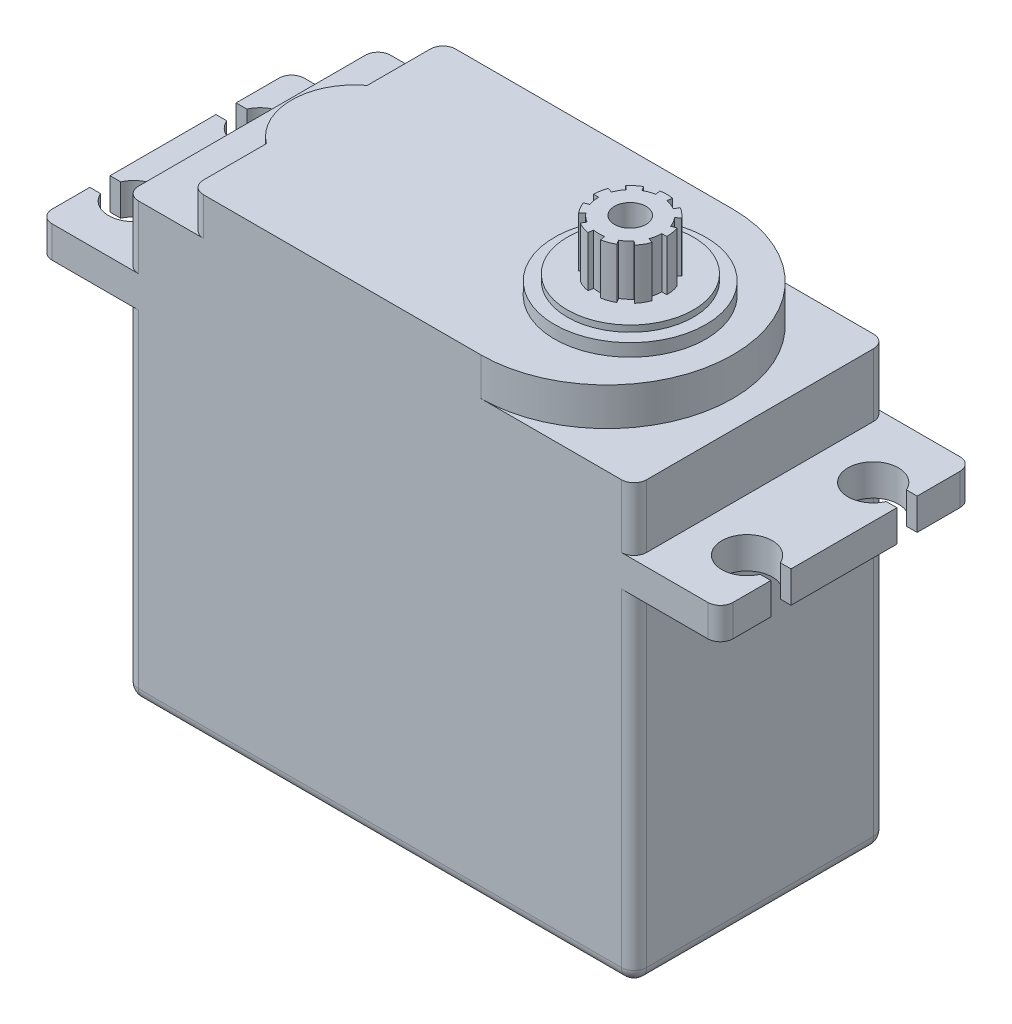
from build123d import *

# Parameters (mm, degrees)
BOSS_EXTRUDE1_DEPTH   = 20
FILLET1_R             = 1
CUT_EXTRUDE1_DEPTH    = 20
SKETCH3_W             = 51.867663345
SKETCH3_H             = 35.261757523
CUT_EXTRUDE2_DEPTH    = 3
SKETCH4_R             = 6
BOSS_EXTRUDE2_DEPTH   = 1
SKETCH5_R             = 5
BOSS_EXTRUDE3_DEPTH   = 0.5
SKETCH6_R             = 1
BOSS_EXTRUDE4_DEPTH   = 4
M3_TAPPED_HOLE1_D     = 2.5
M3_TAPPED_HOLE1_DEPTH = 7.5
M3_TAPPED_HOLE1_TIP   = 0.751075774


with BuildPart() as part:
    # Sketch1 → Boss-Extrude1 (new body)
    with BuildSketch(Plane.XY):
        Polygon((20.15, 8), (27, 8), (27, 10.5), (20.15, 10.5), (20.15, 18.5), (-20.15, 18.5), (-20.15, 10.5), (-27, 10.5), (-27, 8), (-20.15, 8), (-20.15, -19), (20.15, -19), align=None)
    extrude(amount=BOSS_EXTRUDE1_DEPTH)

    # Fillet1
    fillet1_edges = [part.edges().sort_by_distance(p)[0] for p in [
        (-27, 9.25, 20),
        (20.15, 14.5, 0),
        (27, 9.25, 0),
        (20.15, -5.5, 0),
        (0, -19, 0),
        (-20.15, -5.5, 0),
        (-27, 9.25, 0),
        (-20.15, 14.5, 0),
        (-20.15, -5.5, 20),
        (0, -19, 20),
        (-20.15, 18.5, 10),
        (20.15, 18.5, 10),
        (20.15, -19, 10),
        (-20.15, -19, 10),
        (20.15, -5.5, 20),
        (27, 9.25, 20),
        (20.15, 14.5, 20),
        (-20.15, 14.5, 20),
    ]]
    fillet(fillet1_edges, radius=FILLET1_R)

    # Sketch2 → Cut-Extrude1 (cut)
    with BuildSketch(Plane(origin=(0, 10.5, 0), x_dir=(1, 0, 0), z_dir=(0, 1, 0))):
        with BuildLine():
            Line((-26.148030278, -4.4), (-29.222738853, -4.4))
            Line((-29.222738853, -4.4), (-29.222738853, -6))
            Line((-29.222738853, -6), (-26.148030278, -6))
            ThreePointArc((-26.148030278, -6), (-22.315, -5.2), (-26.148030278, -4.4))
        make_face()
        with BuildLine():
            Line((-26.148030278, -14.4), (-29.222738853, -14.4))
            Line((-29.222738853, -14.4), (-29.222738853, -16))
            Line((-29.222738853, -16), (-26.148030278, -16))
            ThreePointArc((-26.148030278, -16), (-22.315, -15.2), (-26.148030278, -14.4))
        make_face()
        with BuildLine():
            Line((26.148030278, -16), (29.222738853, -16))
            Line((29.222738853, -16), (29.222738853, -14.4))
            Line((29.222738853, -14.4), (26.148030278, -14.4))
            ThreePointArc((26.148030278, -14.4), (22.315, -15.2), (26.148030278, -16))
        make_face()
        with BuildLine():
            Line((29.222738853, -4.4), (29.222738853, -6))
            Line((29.222738853, -6), (26.148030278, -6))
            ThreePointArc((26.148030278, -6), (22.315, -5.2), (26.148030278, -4.4))
            Line((26.148030278, -4.4), (29.222738853, -4.4))
        make_face()
    extrude(amount=-CUT_EXTRUDE1_DEPTH, mode=Mode.SUBTRACT)

    # Sketch3 → Cut-Extrude2 (cut)
    with BuildSketch(Plane(origin=(0, 18.5, 0), x_dir=(1, 0, 0), z_dir=(0, 1, 0))):
        with Locations((-0.933831673, -10.85793672)):
            Rectangle(SKETCH3_W, SKETCH3_H)
        with BuildLine():
            Line((-14, 0), (8, 0))
            ThreePointArc((8, 0), (18, -10), (8, -20))
            Line((8, -20), (-14, -20))
            ThreePointArc((-14, -20), (-14.707106781, -19.707106781), (-15, -19))
            Line((-15, -19), (-15, -14))
            ThreePointArc((-15, -14), (-17, -10), (-15, -6))
            Line((-15, -6), (-15, -1))
            ThreePointArc((-15, -1), (-14.707106781, -0.292893219), (-14, 0))
        make_face(mode=Mode.SUBTRACT)
    extrude(amount=-CUT_EXTRUDE2_DEPTH, mode=Mode.SUBTRACT)

    # Sketch4 → Boss-Extrude2 (add)
    with BuildSketch(Plane(origin=(0, 18.5, 0), x_dir=(1, 0, 0), z_dir=(0, 1, 0))):
        with Locations((9.85, -10)):
            Circle(SKETCH4_R)
    extrude(amount=BOSS_EXTRUDE2_DEPTH)

    # Sketch5 → Boss-Extrude3 (add)
    with BuildSketch(Plane(origin=(0, 19.5, 0), x_dir=(1, 0, 0), z_dir=(0, 1, 0))):
        with Locations(Location((9.851314919, -9.987632383, 0), (0, 0, 270))):
            Circle(SKETCH5_R)
    extrude(amount=BOSS_EXTRUDE3_DEPTH)

    # Sketch6 → Boss-Extrude4 (add)
    with BuildSketch(Plane(origin=(0, 20, 0), x_dir=(1, 0, 0), z_dir=(0, 1, 0))):
        with BuildLine():
            Line((10.284120444, -7.537980617), (10.353579715, -7.144057516))
            ThreePointArc((10.353579715, -7.144057516), (9.85, -7.1), (9.346420285, -7.144057516))
            Line((9.346420285, -7.144057516), (9.415879556, -7.537980617))
            ThreePointArc((9.415879556, -7.537980617), (8.994949642, -7.650768448), (8.6, -7.834936491))
            Line((8.6, -7.834936491), (8.4, -7.488526329))
            ThreePointArc((8.4, -7.488526329), (7.985915932, -7.778471115), (7.628471115, -8.135915932))
            Line((7.628471115, -8.135915932), (7.934888892, -8.393030976))
            ThreePointArc((7.934888892, -8.393030976), (7.684936491, -8.75), (7.500768448, -9.144949642))
            Line((7.500768448, -9.144949642), (7.1248914, -9.008141584))
            ThreePointArc((7.1248914, -9.008141584), (6.994057516, -9.496420285), (6.95, -10))
            Line((6.95, -10), (7.35, -10))
            ThreePointArc((7.35, -10), (7.387980617, -10.434120444), (7.500768448, -10.855050358))
            Line((7.500768448, -10.855050358), (7.1248914, -10.991858416))
            ThreePointArc((7.1248914, -10.991858416), (7.338526329, -11.45), (7.628471115, -11.864084068))
            Line((7.628471115, -11.864084068), (7.934888892, -11.606969024))
            ThreePointArc((7.934888892, -11.606969024), (8.243030976, -11.915111108), (8.6, -12.165063509))
            Line((8.6, -12.165063509), (8.4, -12.511473671))
            ThreePointArc((8.4, -12.511473671), (8.858141584, -12.7251086), (9.346420285, -12.855942484))
            Line((9.346420285, -12.855942484), (9.415879556, -12.462019383))
            ThreePointArc((9.415879556, -12.462019383), (9.85, -12.5), (10.284120444, -12.462019383))
            Line((10.284120444, -12.462019383), (10.353579715, -12.855942484))
            ThreePointArc((10.353579715, -12.855942484), (10.841858416, -12.7251086), (11.3, -12.511473671))
            Line((11.3, -12.511473671), (11.1, -12.165063509))
            ThreePointArc((11.1, -12.165063509), (11.456969024, -11.915111108), (11.765111108, -11.606969024))
            Line((11.765111108, -11.606969024), (12.071528885, -11.864084068))
            ThreePointArc((12.071528885, -11.864084068), (12.361473671, -11.45), (12.5751086, -10.991858416))
            Line((12.5751086, -10.991858416), (12.199231552, -10.855050358))
            ThreePointArc((12.199231552, -10.855050358), (12.312019383, -10.434120444), (12.35, -10))
            Line((12.35, -10), (12.75, -10))
            ThreePointArc((12.75, -10), (12.705942484, -9.496420285), (12.5751086, -9.008141584))
            Line((12.5751086, -9.008141584), (12.199231552, -9.144949642))
            ThreePointArc((12.199231552, -9.144949642), (12.015063509, -8.75), (11.765111108, -8.393030976))
            Line((11.765111108, -8.393030976), (12.071528885, -8.135915932))
            ThreePointArc((12.071528885, -8.135915932), (11.714084068, -7.778471115), (11.3, -7.488526329))
            Line((11.3, -7.488526329), (11.1, -7.834936491))
            ThreePointArc((11.1, -7.834936491), (10.705050358, -7.650768448), (10.284120444, -7.537980617))
        make_face()
        with Locations(Location((9.85, -10, 0), (0, 0, 270))):
            Circle(SKETCH6_R, mode=Mode.SUBTRACT)
    extrude(amount=BOSS_EXTRUDE4_DEPTH)

    # M3 Tapped Hole1
    with Locations(Plane(origin=(9.85, 24, 10), x_dir=(0, 0, 1), z_dir=(0, 1, 0))):
        with Locations((0, 0)):
            Hole(M3_TAPPED_HOLE1_D / 2, depth=M3_TAPPED_HOLE1_DEPTH)
            with Locations((0, 0, -(M3_TAPPED_HOLE1_DEPTH + M3_TAPPED_HOLE1_TIP / 2))):  # 118° drill point
                Cone(0, M3_TAPPED_HOLE1_D / 2, M3_TAPPED_HOLE1_TIP, mode=Mode.SUBTRACT)


solid = part.part
